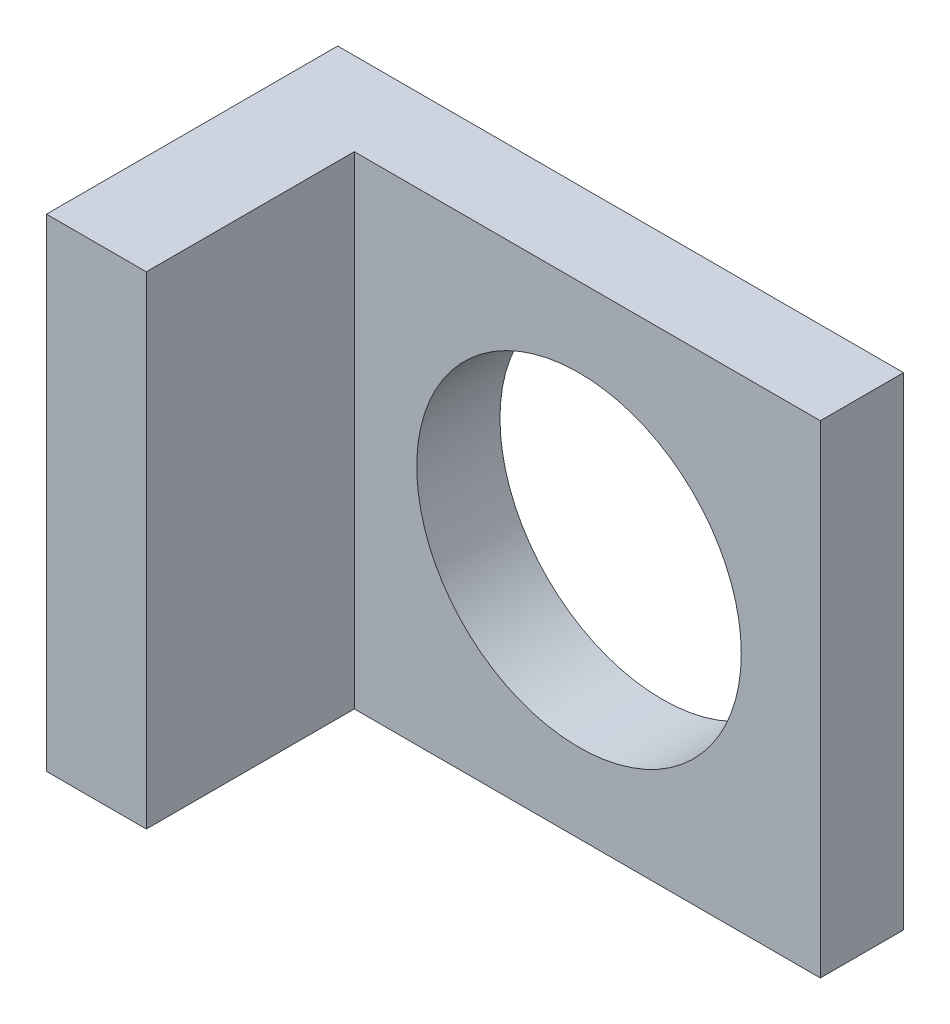
from build123d import *

# Parameters (mm, degrees)
SKETCH_1_W          = 68
SKETCH_1_H          = 58
EXTRUDE_1_DEPTH     = 10
CUT_EXTRUDE_1_REACH = 91.933
SKETCH_2_R          = 19.5
SKETCH_4_W          = 12
SKETCH_4_H          = 58
EXTRUDE_3_DEPTH     = 25


with BuildPart() as part:
    # 草图1 → 凸台-拉伸1 (new body)
    with BuildSketch(Plane.XY):
        with Locations((34, 29)):
            Rectangle(SKETCH_1_W, SKETCH_1_H)
    extrude(amount=EXTRUDE_1_DEPTH)

    # 草图2 → 切除-拉伸1 (cut, up to next)
    with BuildSketch(Plane.XY.offset(10), mode=Mode.PRIVATE) as cut_extrude_1_sk1:
        with Locations((39, 29)):
            Circle(SKETCH_2_R)
    cut_extrude_1_tool1 = extrude(cut_extrude_1_sk1.sketch, amount=-CUT_EXTRUDE_1_REACH, mode=Mode.PRIVATE) & part.part
    add(cut_extrude_1_tool1.solids().sort_by_distance((39, 29, 10))[0], mode=Mode.SUBTRACT)

    # 草图4 → 凸台-拉伸3 (add)
    with BuildSketch(Plane.XY.offset(10)):
        with Locations((6, 29)):
            Rectangle(SKETCH_4_W, SKETCH_4_H)
    extrude(amount=EXTRUDE_3_DEPTH)


solid = part.part
